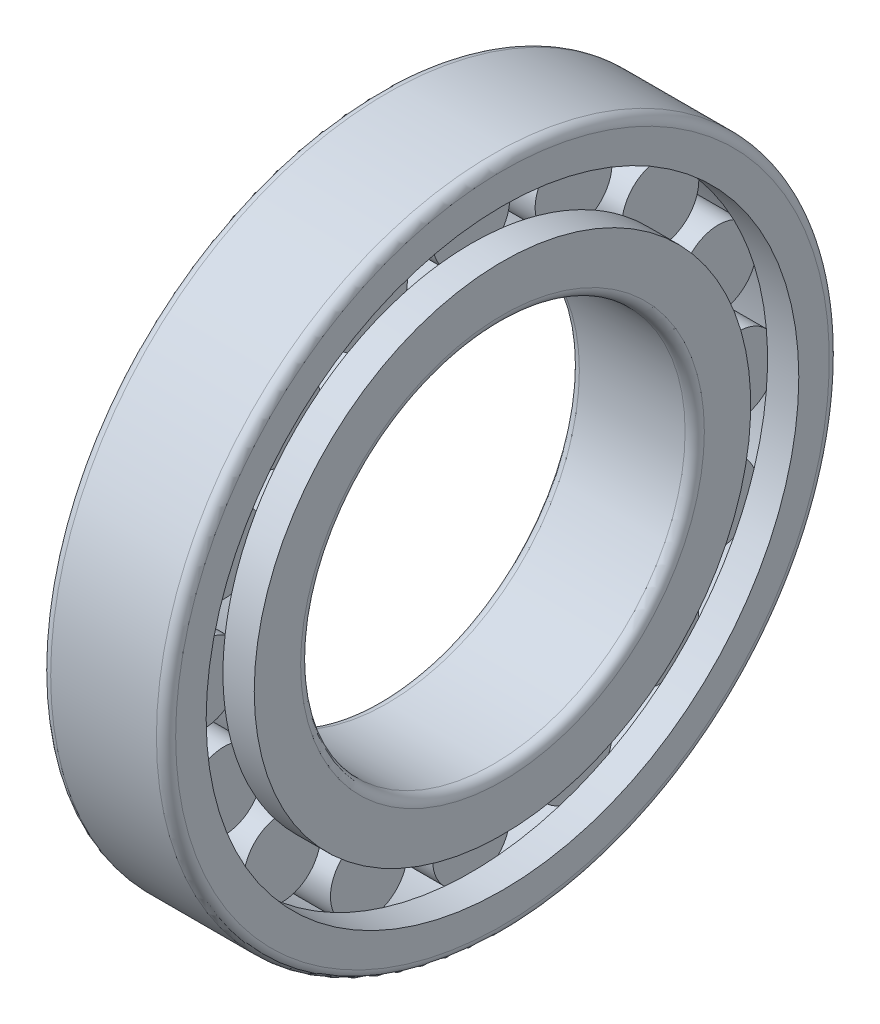
from build123d import *

# Parameters (mm, degrees)
SKETCH_3_W               = 13
SKETCH_3_H               = 8.0001
PATTERN_CIRCULAR_1_COUNT = 16


with BuildPart() as part:
    # 草图2 → Revolve 707 (revolve)
    with BuildSketch(Plane.XY, mode=Mode.PRIVATE) as revolve_707_sk:
        with BuildLine():
            Line((6.5, 47.65), (19.5, 47.65))
            Line((19.5, 47.65), (19.5, 51.65))
            Line((19.5, 51.65), (26, 51.65))
            Line((26, 51.65), (26, 42))
            ThreePointArc((26, 42), (25.414213562, 40.585786438), (24, 40))
            Line((24, 40), (2, 40))
            ThreePointArc((2, 40), (0.585786438, 40.585786438), (0, 42))
            Line((0, 42), (0, 51.65))
            Line((0, 51.65), (6.5, 51.65))
            Line((6.5, 51.65), (6.5, 47.65))
        make_face()
    revolve(revolve_707_sk.sketch.rotate(Axis((-10.080094127, 0, 0), (1, 0, 0)), 90), axis=Axis((-10.080094127, 0, 0), (1, 0, 0)))

    # 草图3 → 凸台-旋转1 (revolve)
    with BuildSketch(Plane.XY):
        with Locations((13, 51.64995)):
            Rectangle(SKETCH_3_W, SKETCH_3_H)
    revolve_1 = revolve(axis=Axis((-1.603948851, 55.65, 0), (1, 0, 0)))

    # 草图4 → 凸台-旋转2 (revolve)
    with BuildSketch(Plane.XY, mode=Mode.PRIVATE) as revolve_2_sk:
        with BuildLine():
            Line((19.5, 61.65), (26, 61.65))
            Line((26, 61.65), (26, 68))
            ThreePointArc((26, 68), (25.414213562, 69.414213562), (24, 70))
            Line((24, 70), (2, 70))
            ThreePointArc((2, 70), (0.585786438, 69.414213562), (0, 68))
            Line((0, 68), (0, 61.65))
            Line((0, 61.65), (6.5, 61.65))
            Line((6.5, 61.65), (6.5, 63.65))
            Line((6.5, 63.65), (19.5, 63.65))
            Line((19.5, 63.65), (19.5, 61.65))
        make_face()
    revolve(revolve_2_sk.sketch.rotate(Axis((0, 0, 0), (1, 0, 0)), 90), axis=Axis((0, 0, 0), (1, 0, 0)))

    # 阵列(圆周)1: 凸台-旋转1 ×16 about axis
    pattern_circular_1_axis = Axis((0, 0, 0), (1, 0, 0))
    for i in range(1, PATTERN_CIRCULAR_1_COUNT):
        add(revolve_1.rotate(pattern_circular_1_axis, i * 360 / PATTERN_CIRCULAR_1_COUNT))


solid = part.part
